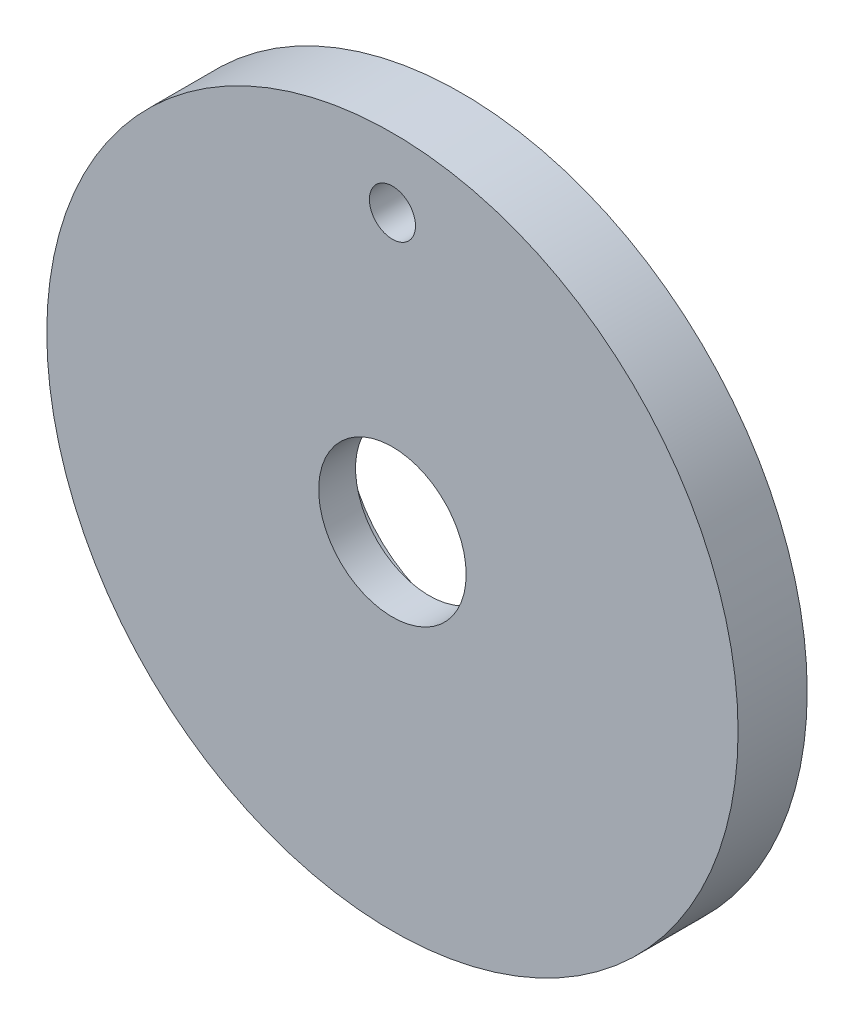
from build123d import *

# Parameters (mm, degrees)
SKETCH_1_R          = 75
SKETCH_1_R_2        = 5
SKETCH_1_R_3        = 16
EXTRUDE_1_DEPTH     = 15
CUT_EXTRUDE_START   = -15
SKETCH_2_R          = 25
CUT_EXTRUDE_1_DEPTH = 7


with BuildPart() as part:
    # 草图1 → 凸台-拉伸1 (new body)
    with BuildSketch(Plane.XY):
        Circle(SKETCH_1_R)
        with Locations((0, 60)):
            Circle(SKETCH_1_R_2, mode=Mode.SUBTRACT)
        Circle(SKETCH_1_R_3, mode=Mode.SUBTRACT)
    extrude(amount=EXTRUDE_1_DEPTH)

    # 草图2 → 切除-拉伸1 (cut)
    with BuildSketch(Plane.XY.offset(15).offset(CUT_EXTRUDE_START)):
        Circle(SKETCH_2_R)
    extrude(amount=CUT_EXTRUDE_1_DEPTH, mode=Mode.SUBTRACT)


solid = part.part
